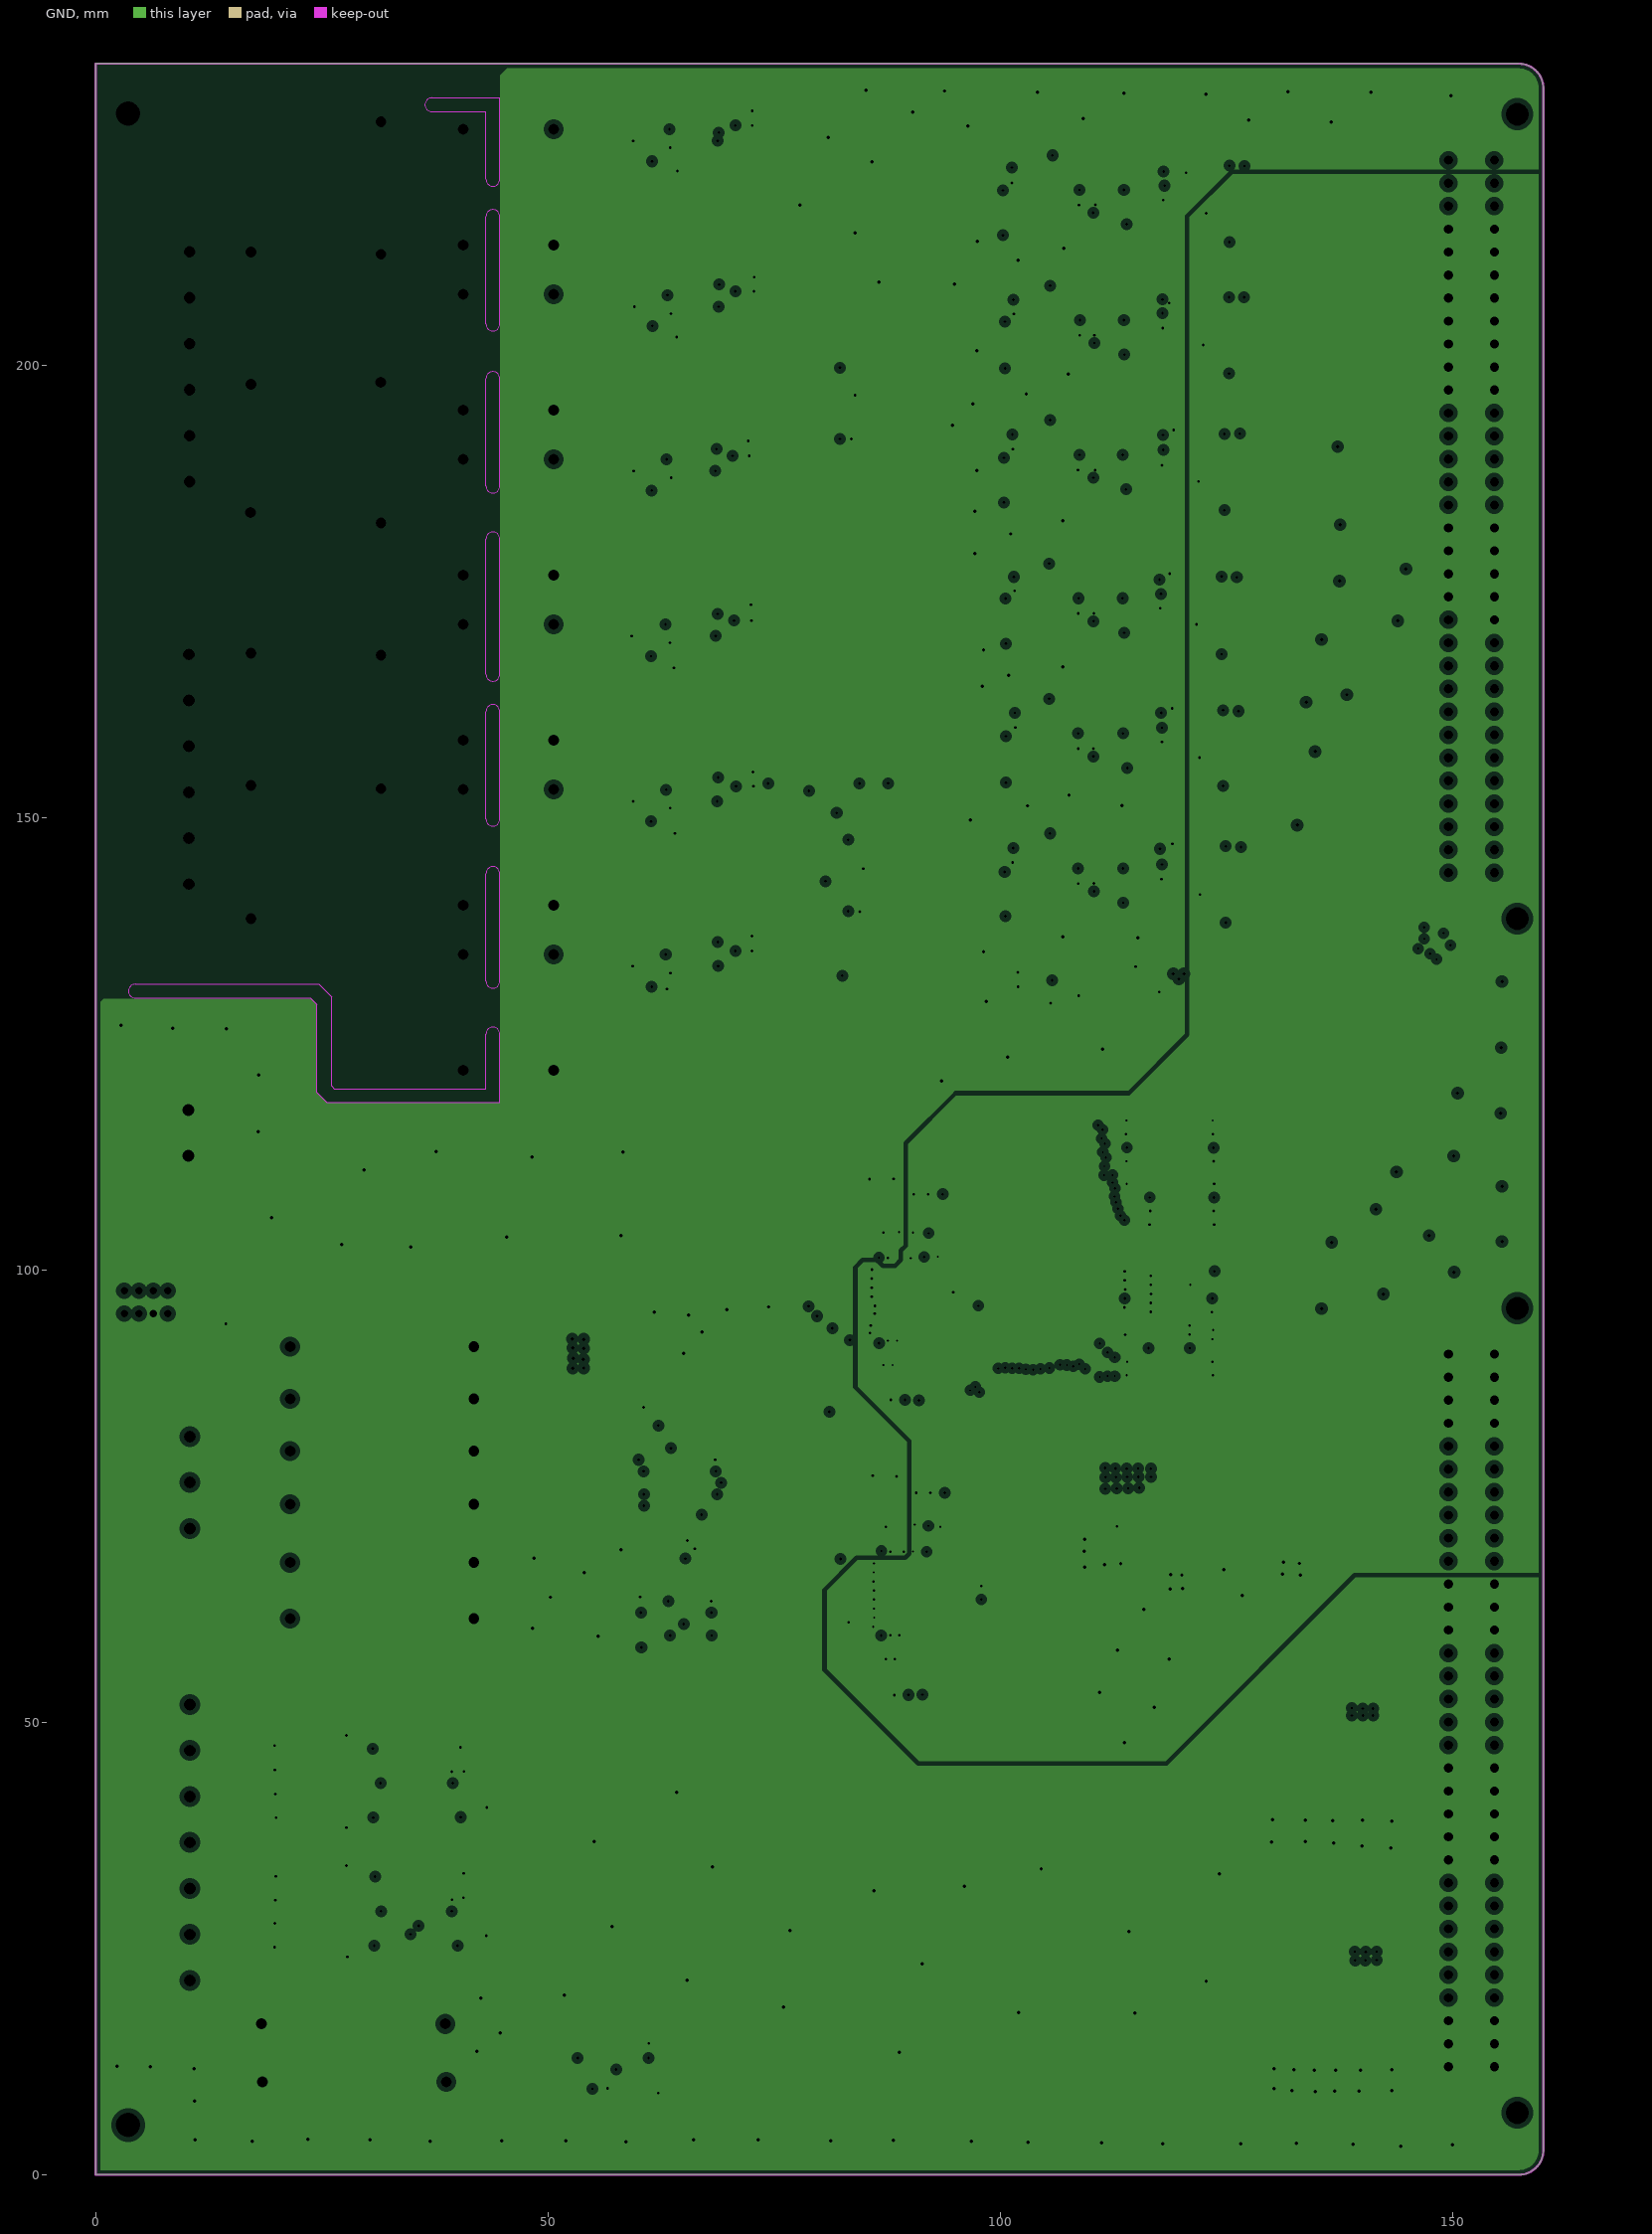
[diagram p0: GND, clearances drawn from the general rule]
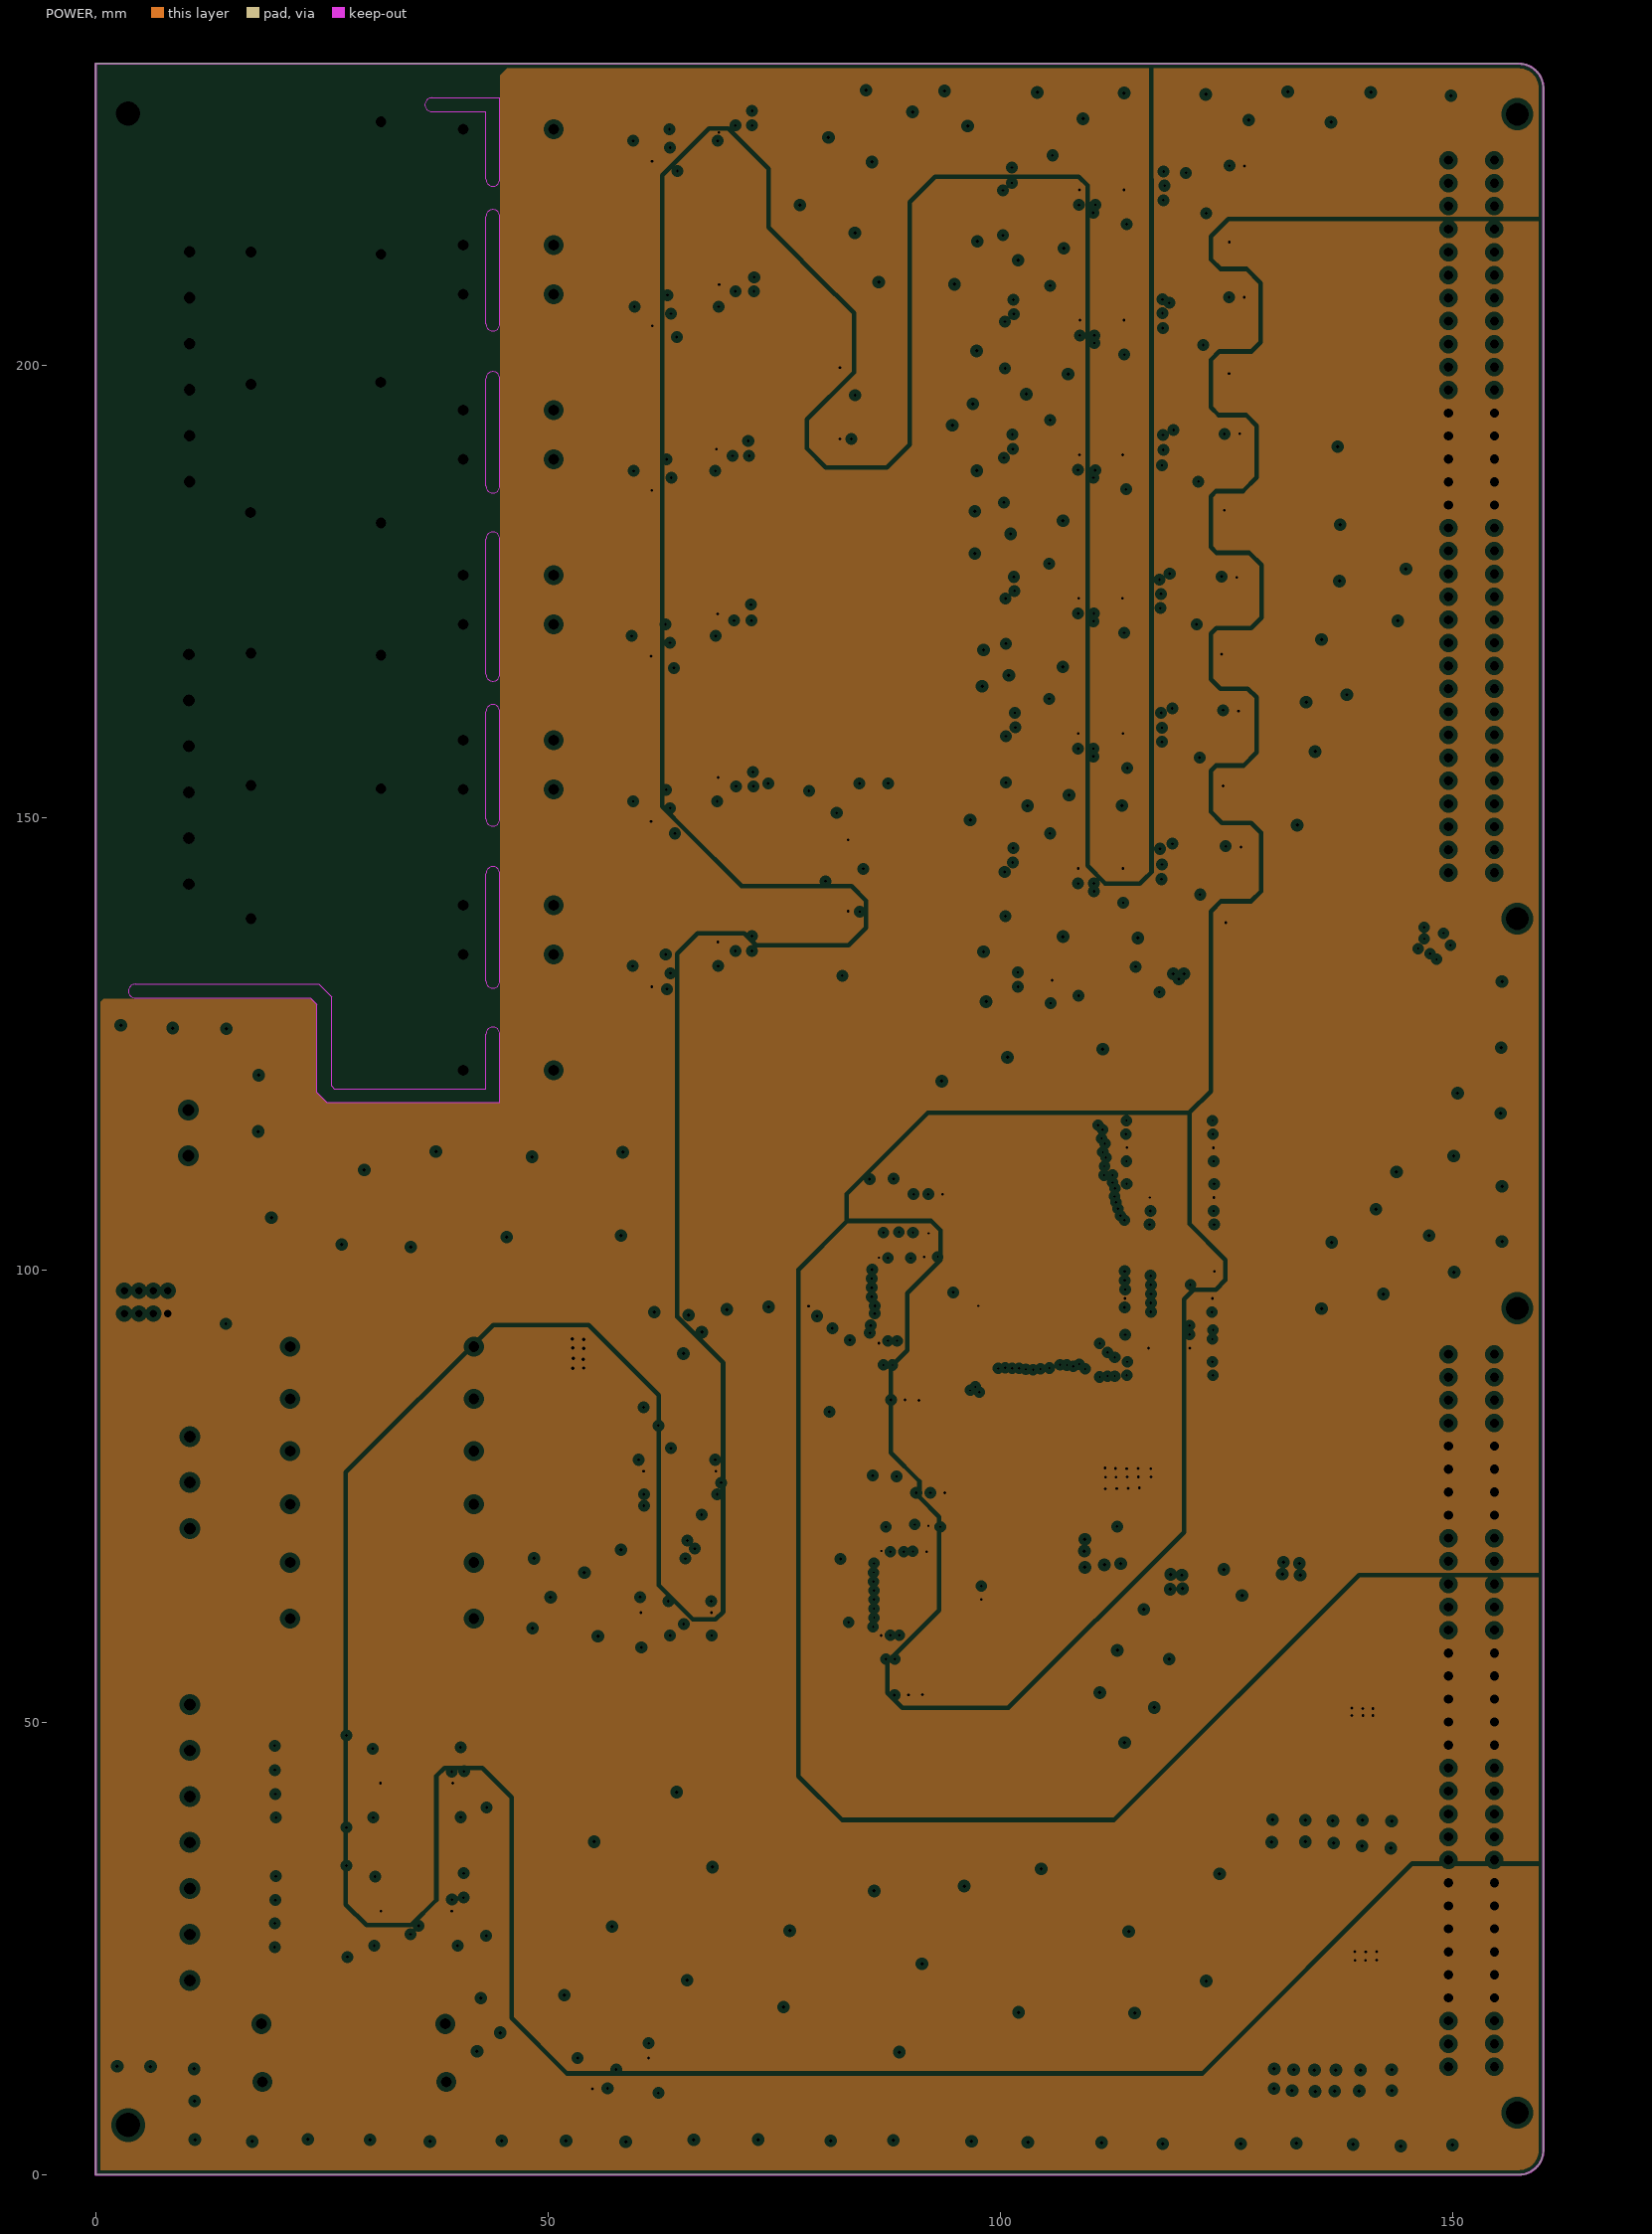
[diagram p1: POWER, clearances drawn from the general rule]
# Altium PCB MISC80584.PCBDoc (part 2 of 7)
## Components (designator, comment, footprint, x,y, rotation, side; value= is the part's Value field where it differs from the comment) (continued)
R111 "5.1k_1%" 0603 65.786,206.477 r90 bottom
R113 "5.1k" 0603 71.628,208.153 r180 bottom
R117 "10k" 0603 103.759,187.985 r270 bottom
R118 "5.1k" 0603 71.653,226.492 r180 bottom
R119 "5.1k_1%" 0603 67.488,224.79 r90 bottom
R120 "5.1k_1%" 0603 65.938,224.815 r90 bottom
R124 "5.1k" 0603 71.628,135.255 r180 bottom
R125 "5.1k_1%" 0603 67.335,133.604 r90 bottom
R126 "5.1k_1%" 0603 65.634,133.604 r90 bottom
R130 "5.1k" 0603 71.679,153.467 r180 bottom
R131 "5.1k_1%" 0603 65.837,151.816 r90 bottom
R132 "10k" 0603 101.879,217.576 r270 bottom
R133 "5.1k_1%" 0603 67.386,151.816 r90 bottom
R137 "5.1k" 0603 71.425,171.78 r180 bottom
R138 "5.1k_1%" 0603 65.659,170.078 r90 bottom
R139 "5.1k_1%" 0603 67.259,170.078 r90 bottom
R145 "50kΩ_2W_1%" AXIAL0.8 31.547,182.55 r225 top
R146 "10k" 0603 102.133,203.022 r270 bottom
R147 "10k" 0603 102.032,187.985 r270 bottom
R150 "10k" 0603 115.367,221.412 r0 top
R151 "10k" 0603 115.265,207.264 r0 top
R152 "10k" 0603 115.341,192.278 r0 top
R155 "10k" 0603 115.392,219.837 r0 top
R156 "10k" 0603 115.265,205.74 r0 top
R157 "10k" 0603 115.341,190.627 r0 top
R161 "50kΩ_2W_1%" AXIAL0.8 31.547,167.919 r225 top
R162 "10k" 0603 116.992,223.164 r180 top
R165 "50kΩ_2W_1%" AXIAL0.8 31.547,153.187 r225 top
R168 "50kΩ_2W_1%" AXIAL0.8 31.547,226.873 r225 top
R171 "50kΩ_2W_1%" AXIAL0.8 31.547,212.242 r225 top
R174 "50kΩ_2W_1%" AXIAL0.8 31.496,198.095 r225 top
R211 "10k" 0603 116.942,208.788 r180 top
R224 "0" 0603 104.445,129.667 r180 top
R225 "10k" 0603 117.018,193.904 r180 top
R339 "3.3k" 0603 11.887,98.755 r0 top
R340 "10k" 0603 11.862,95.606 r0 top
R341 "10k" 0603 11.836,94.082 r0 top
R342 "3.3k" 0603 11.862,97.18 r0 top
R349 "10k" 0603 104.089,176.606 r180 top
R350 "10k" 0603 104.191,161.569 r180 top
R351 "10k" 0603 103.962,146.634 r180 top
R353 "10k" 0603 102.413,178.181 r0 top
R354 "10k" 0603 102.489,163.17 r0 top
R355 "10k" 0603 102.286,148.209 r0 top
R357 "10k" 0603 100.584,170.84 r90 bottom
R358 "10k" 0603 100.609,155.346 r90 bottom
R359 "10k" 0603 100.482,140.716 r90 bottom
R360 "10k" 0603 107.112,176.378 r90 bottom
R361 "10k" 0603 107.163,161.493 r90 bottom
R362 "10k" 0603 107.112,146.533 r90 bottom
R364 "10k" 0603 102.26,172.466 r270 bottom
R365 "10k" 0603 102.311,156.997 r270 bottom
R366 "10k" 0603 103.835,142.392 r270 bottom
R372 "10k" 0603 104.013,172.466 r270 bottom
R373 "10k" 0603 104.013,157.023 r270 bottom
R374 "10k" 0603 102.159,142.392 r270 bottom
R375 "10k" 0603 115.138,176.301 r0 top
R376 "10k" 0603 115.138,161.595 r0 top
R377 "10k" 0603 115.164,146.558 r0 top
R379 "10k" 0603 115.138,174.727 r0 top
R380 "10k" 0603 115.164,159.944 r0 top
R381 "10k" 0603 115.189,144.831 r0 top
R382 "10k" 0603 116.764,178.003 r180 top
R383 "10k" 0603 116.815,163.17 r180 top
R384 "10k" 0603 116.815,148.184 r180 top
R399 "5.1k" 0603 103.835,220.142 r180 top
R400 "5.1k" 0603 104.038,205.664 r180 top
R401 "5.1k" 0603 103.937,190.729 r180 top
R414 "5.1k" 0603 71.374,189.992 r180 bottom
R423 "5.1k" 0603 104.089,175.057 r180 top
R430 "5.1k" 0603 104.165,159.969 r180 top
R431 "5.1k" 0603 103.988,145.034 r180 top
R435 "2.4k" 0603 115.341,188.951 r0 top
R437 "2.4k" 0603 115.367,218.237 r0 top
R438 "2.4k" 0603 115.316,204.089 r0 top
R444 "2.4k" 0603 115.113,173.152 r0 top
R445 "2.4k" 0603 115.189,158.369 r0 top
R446 "2.4k" 0603 115.189,143.205 r0 top
R450 "5.6k" 0603 115.367,216.586 r0 top
R451 "5.6k" 0603 115.392,202.286 r0 top
R452 "5.6k" 0603 115.367,187.325 r0 top
R459 "5.6k" 0603 115.164,169.977 r0 top
R460 "5.6k" 0603 115.189,156.718 r0 top
R461 "5.6k" 0603 115.214,141.605 r0 top
R486 "2k" 0603 127,220.878 r180 bottom
R487 "2k" 0603 126.949,206.223 r180 bottom
R488 "2k" 0603 126.467,191.186 r180 bottom
R491 "2k" 0603 125.451,223.037 r180 top
R492 "2k" 0603 125.451,208.763 r180 top
R493 "2k" 0603 125.07,193.726 r180 top
R503 "2k" 0603 126.136,175.438 r180 bottom
R506 "2k" 0603 126.314,160.655 r180 bottom
R507 "2k" 0603 126.594,145.567 r180 bottom
R510 "2k" 0603 124.511,177.825 r180 top
R511 "2k" 0603 124.638,163.093 r180 top
R512 "2k" 0603 124.739,148.158 r180 top
R591 "10k" 0603 121.971,216.789 r270 top
R592 "10k" 0603 121.615,202.235 r270 top
R593 "10k" 0603 120.802,187.147 r270 top
R600 "10k" 0603 120.777,171.348 r270 top
R601 "10k" 0603 121.133,156.642 r270 top
R602 "10k" 0603 121.26,141.503 r270 top
R605 "4.7k" 0603 91.008,88.265 r270 top
R607 "4.7k" 0603 89.459,88.265 r270 top
R608 "4.7k" 0603 87.909,88.265 r270 top
R609 "4.7k" 0603 91.389,55.753 r270 top
R611 "4.7k" 0603 89.84,55.753 r270 top
R612 "4.7k" 0603 88.29,55.753 r270 top
SPT1 "SPT204A" SPT204A 40.615,158.547 r0 top
SPT2 "SPT204A" SPT204A 40.64,140.31 r0 top
SPT3 "SPT204A" SPT204A 40.64,122.072 r0 top
SPT4 "SPT204A" SPT204A 40.615,213.258 r0 top
SPT5 "SPT204A" SPT204A 40.64,195.021 r0 top
SPT6 "SPT204A" SPT204A 40.64,176.784 r0 top
U1 "AD7606" AD7606_LQFP64 86.589,90.805 r90 top
U2 "AD7606" AD7606_LQFP64 86.843,58.344 r90 top
U3 "SN74LVCH16T245_TSSOP48" SN74LVC16245_TSSOP48 115.214,105.029 r0 top
U4 "SN74LVCH16T245_TSSOP48" SN74LVC16245_TSSOP48 122.25,99.873 r180 top
U5 "TL064I" TL064D_SOIC-14 64.16,62.154 r0 top
U6 "TL064I" TL064D_SOIC-14 109.626,219.38 r0 top
U7 "TL064I" TL064D_SOIC-14 109.652,204.978 r0 top
U8 "TL064I" TL064D_SOIC-14 109.525,190.094 r0 top
U9 "TL061D" TL061_SOIC8 57.277,12.294 r0 top
U15 "TL064I" TL064D_SOIC-14 109.525,174.244 r0 top
U16 "TL064I" TL064D_SOIC-14 109.525,159.309 r0 top
U17 "TL064I" TL064D_SOIC-14 109.525,144.399 r0 top
U20 "TL064I" TL064D_SOIC-14 35.382,29.159 r0 top
U26 "OP07CS" SO-8 61.392,172.618 r0 top
U27 "OP07CS" SO-8 61.392,154.356 r0 top
U31 "OP07CS" SO-8 61.468,136.144 r0 top
U32 "OP07CS" SO-8 61.519,227.33 r0 top
U35 "OP07CS" SO-8 61.544,209.017 r0 top
U36 "OP07CS" SO-8 61.468,190.856 r0 top
U37 "TL064I" TL064D_SOIC-14 83.185,143.586 r270 top
U38 "TL064I" TL064D_SOIC-14 82.271,195.834 r270 top
U39 "TL064I" TL064D_SOIC-14 35.408,43.307 r0 top
U40 "TL064I" TL064D_SOIC-14 64.592,77.775 r0 top
U44 "REF195" SO-8 107.036,133.299 r0 top
U45 "AS1117-3.3V" SOT223 132.182,69.926 r90 top
UIN4 "TLP285" TLP285_SOP4 125.324,220.701 r270 top
UIN5 "TLP285" TLP285_SOP4 125.273,206.146 r270 top
UIN6 "TLP285" TLP285_SOP4 124.765,191.059 r270 top
UIN13 "TLP285" TLP285_SOP4 124.46,175.26 r270 top
UIN14 "TLP285" TLP285_SOP4 124.638,160.553 r270 top
UIN15 "TLP285" TLP285_SOP4 124.917,145.44 r270 top

## Footprints (in the part's own frame and the unit in brackets; to place one, negate y for a bottom-side part, rotate by r counter-clockwise, add the part's x,y. Pads: shape width x height; smd on the part's side, far side on the other; paste and mask are expansions set on the pad)
1N4148-A [mil]
  rect 60x50 smd: A(0,0) K(124,0)
  silkscreen extent -38,-45 162,45
0603 [mil]
  rect 25x32 smd: 1(0,0) 2(66,0)
  silkscreen extent -22,-25 88,25
0805 [mil]
  rect 60x50 smd: 1(0,0) 2(90,0)
  silkscreen extent -50,-45 140,45
3528_CASE-B [mil]
  rect 75x90 smd: 1(0,0) 2(135,0)
  silkscreen extent -65,-65 195,65
7343_CASE-D [mm]
  rect 2.4x3 smd: 1(3.12,0) 2(-3.12,0)
  silkscreen extent -4.65,-2.5 5.1,2.5
AD7606_LQFP64 [mil]
  oval 60x10 smd: 1(0,0)
  rect 60x10 smd: 2(0,-19.69) 3(0,-39.37) 4(0,-59.06) 5(0,-78.74) 6(0,-98.43) 7(0,-118.11) 8(0,-137.8) 9(0,-157.48) 10(0,-177.17) 11(0,-196.85) 12(0,-216.54) 13(0,-236.22) 14(0,-255.91) 15(0,-275.59) 16(0,-295.28) 33(472.44,-295.28) 34(472.44,-275.59) 35(472.44,-255.91) 36(472.44,-236.22) 37(472.44,-216.54) 38(472.44,-196.85) 39(472.44,-177.17) 40(472.44,-157.48) 41(472.44,-137.8) 42(472.44,-118.11) 43(472.44,-98.43) 44(472.44,-78.74) 45(472.44,-59.06) 46(472.44,-39.37) 47(472.44,-19.69) 48(472.44,0)
  rect 10x60 smd: 17(88.58,-383.86) 18(108.27,-383.86) 19(127.95,-383.86) 20(147.64,-383.86) 21(167.32,-383.86) 22(187.01,-383.86) 23(206.69,-383.86) 24(226.38,-383.86) 25(246.06,-383.86) 26(265.75,-383.86) 27(285.43,-383.86) 28(305.12,-383.86) 29(324.8,-383.86) 30(344.49,-383.86) 31(364.17,-383.86) 32(383.86,-383.86) 49(383.86,88.58) 50(364.17,88.58) 51(344.49,88.58) 52(324.8,88.58) 53(305.12,88.58) 54(285.43,88.58) 55(265.75,88.58) 56(246.06,88.58) 57(226.38,88.58) 58(206.69,88.58) 59(187.01,88.58) 60(167.32,88.58) 61(147.64,88.58) 62(127.95,88.58) 63(108.27,88.58) 64(88.58,88.58)
  silkscreen extent 39,-344 433,49
AXIAL0.8 [mm]
  round 2 hole 1.2: 1(-0.009,-0.012) 2(20.311,-0.012)
  silkscreen extent 1.26,-2.04 19.04,2.02
BUS64W-A [mil]
  round 200 hole 100: 0(-200,100) 0(3300,100)
  rect 60x60 hole 40: A1(0,0)
  round 60 hole 40: A2(100,0) A3(200,0) A4(300,0) A5(400,0) A6(500,0) A7(600,0) A8(700,0) A9(800,0) A10(900,0) A11(1000,0) A12(1100,0) A13(1200,0) A14(1300,0) A15(1400,0) A16(1500,0) A17(1600,0) A18(1700,0) A19(1800,0) A20(1900,0) A21(2000,0) A22(2100,0) A23(2200,0) A24(2300,0) A25(2400,0) A26(2500,0) A27(2600,0) A28(2700,0) A29(2800,0) A30(2900,0) A31(3000,0) A32(3100,0) C1(0,-200) C2(100,-200) C3(200,-200) C4(300,-200) C5(400,-200) C6(500,-200) C7(600,-200) C8(700,-200) C9(800,-200) C10(900,-200) C11(1000,-200) C12(1100,-200) C13(1200,-200) C14(1300,-200) C15(1400,-200) C16(1500,-200) C17(1600,-200) C18(1700,-200) C19(1800,-200) C20(1900,-200) C21(2000,-200) C22(2100,-200) C23(2200,-200) C24(2300,-200) C25(2400,-200) C26(2500,-200) C27(2600,-200) C28(2700,-200) C29(2800,-200) C30(2900,-200) C31(3000,-200) C32(3100,-200)
  silkscreen extent -300,-250 3400,500
EDGCON_2p_5.08mm_ear [mil]
  round 100 hole 51: 1(-200,0) 2(0,0)
  silkscreen extent -500,-400 300,80
EDGCON_3p_5.08mm_ear [mil]
  round 100 hole 51: 1(-200,0) 2(0,0) 3(200,0)
  silkscreen extent -500,-400 500,80
EDGCon_6P_5.08mm_ear [mil]
  round 100 hole 51: 1(0,0) 2(200,0) 3(400,0) 4(600,0) 5(800,0) 6(1000,0)
  silkscreen extent -300,-400 1300,80
EDGCon_7P_5.08mm_ear [mil]
  round 100 hole 51: 1(0,0) 2(200,0) 3(400,0) 4(600,0) 5(800,0) 6(1000,0) 7(1200,0)
  silkscreen extent -300,-400 1500,80
L470UF [mil]
  rect 55x120 smd: 1(0,219) 2(0,-10)
  silkscreen extent -138,-33 138,242
LEDGroup_4 [mil]
  oval 45x55 hole 32: 1(0,100) 2(0,0) 3(62.99,100) 4(62.99,0) 5(125.98,100) 6(125.98,0) 7(188.98,100) 8(188.98,0)
  silkscreen extent -244,-45 249,145
SN74LVC16245_TSSOP48 [mm]
  oval 1.5x0.3 smd: 1(0,11.5) 2(0,11) 3(0,10.5) 4(0,10) 5(0,9.5) 6(0,9) 7(0,8.5) 8(0,8) 9(0,7.5) 10(0,7) 11(0,6.5) 12(0,6) 13(0,5.5) 14(0,5) 15(0,4.5) 16(0,4) 17(0,3.5) 18(0,3) 19(0,2.5) 20(0,2) 21(0,1.5) 22(0,1) 23(0,0.5) 24(0,0) 25(7.1,0) 26(7.1,0.5) 27(7.1,1) 28(7.1,1.5) 29(7.1,2) 30(7.1,2.5) 31(7.1,3) 32(7.1,3.5) 33(7.1,4) 34(7.1,4.5) 35(7.1,5) 36(7.1,5.5) 37(7.1,6) 38(7.1,6.5) 39(7.1,7) 40(7.1,7.5) 41(7.1,8) 42(7.1,8.5) 43(7.1,9) 44(7.1,9.5) 45(7.1,10) 46(7.1,10.5) 47(7.1,11) 48(7.1,11.5)
  silkscreen extent 1.02,-0.5 6.1,12
SO-8 [mil]
  oval 80x24 smd: 1(0,0) 2(0,-50) 3(0,-100) 4(0,-150) 5(220,-150) 6(220,-100) 7(220,-50) 8(220,0)
  silkscreen extent 60,-175 160,25
SOT23-3 [mil]
  rect 36x36 smd: B(-125,-85) E(-50,-85)
  rect 36x40 smd: C(-87,0)
  silkscreen extent -145,-90 -30,0
SOT23R [mil]
  rect 36x36 smd: 1(0,0) 2(75,0)
  rect 36x50 smd: 3(38,80)
  silkscreen extent -20,-5 95,85
SOT223 [mil]
  rect 59x79 smd: 1(0,0) 2(90,0) 3(181,0)
  rect 150x79 smd: 2(90,254)
  silkscreen extent -49,52 231,202
SPT204A [mm]
  round 2 hole 1.2: 0(0,12.8) 1(0,0) 2(10,0) 3(10,12.8)
  silkscreen extent -5.08,-2.54 15.24,15.24
TL061_SOIC8 [mm]
  oval 1.9x0.6 smd: 1(-2.35,1.905) 2(-2.35,0.635) 3(-2.35,-0.635) 4(-2.35,-1.905) 5(2.35,-1.905) 6(2.35,-0.635) 7(2.35,0.635) 8(2.35,1.905)
  silkscreen extent -2.47,-2.5 1,2.88
TL064D_SOIC-14 [mm]
  oval 2.2x0.6 smd: 1(-2.4,3.81) 2(-2.4,2.54) 3(-2.4,1.27) 4(-2.4,0) 5(-2.4,-1.27) 6(-2.4,-2.54) 7(-2.4,-3.81) 8(2.4,-3.81) 9(2.4,-2.54) 10(2.4,-1.27) 11(2.4,0) 12(2.4,1.27) 13(2.4,2.54) 14(2.4,3.81)
  silkscreen extent -2.52,-4.4 0.9,4.78
TLP285_SOP4 [mil]
  oval 80x24 smd: 1(0,0) 2(0,-50) 3(220,-50) 4(220,0)
  silkscreen extent 60,-80 160,25